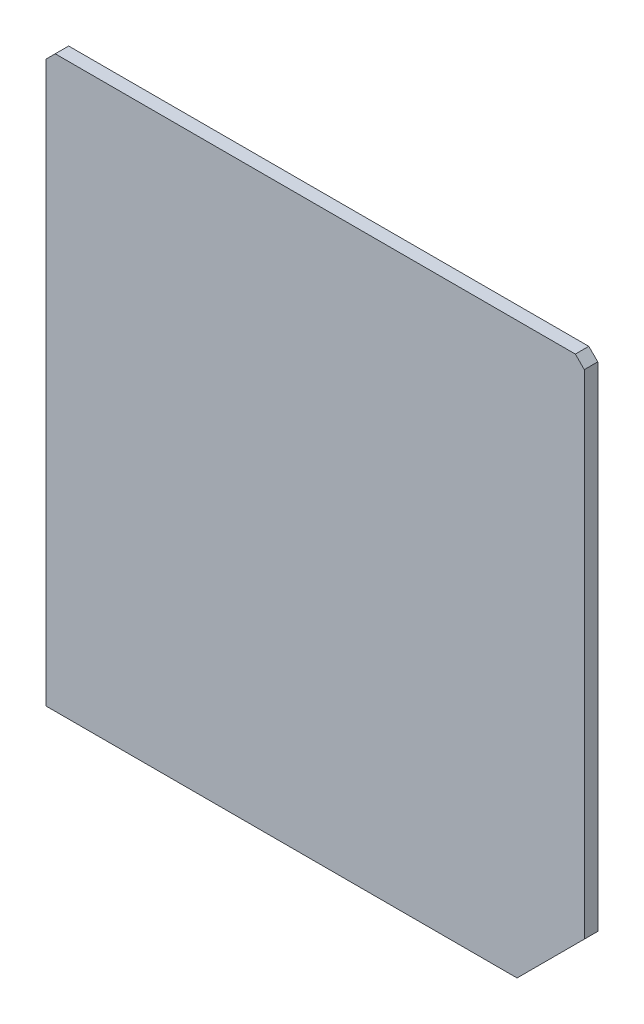
SolidWorks part; units mm, degrees
material "1023 Carbon Steel Plate (SS)"
ref_plane "Front Plane" through (0, 0, 0) normal (0, 0, 1) x (1, 0, 0)
ref_plane "Top Plane" through (0, 0, 0) normal (0, 1, 0) x (1, 0, 0)
ref_plane "Right Plane" through (0, 0, 0) normal (1, 0, 0) x (0, 0, -1)
sketch "Sketch1" plane through (0, 0, 0) normal (0, 0, 1) x (1, 0, 0)
  line L1 (60, 63.5) -> (-60, 63.5)
  line L2 (60, 63.5) -> (60, -63.5)
  line L3 (60, -63.5) -> (-60, -63.5)
  line L4 (-60, 63.5) -> (-60, -63.5)
  line L5 (60, 63.5) -> (-60, -63.5) construction
  line L6 (60, -63.5) -> (-60, 63.5) construction
  point P0 (0, 0)
  dimension "D1" = 120
  dimension "D2" = 127
extrude "Boss-Extrude1" add sketch "Sketch1" along normal blind 3
chamfer "Chamfer1" distance 15 angle 45 1 edges at (60, -63.5, 1.5)
chamfer "Chamfer2" distance 2 angle 45 2 edges at (60, 63.5, 1.5) (-60, 63.5, 1.5)
